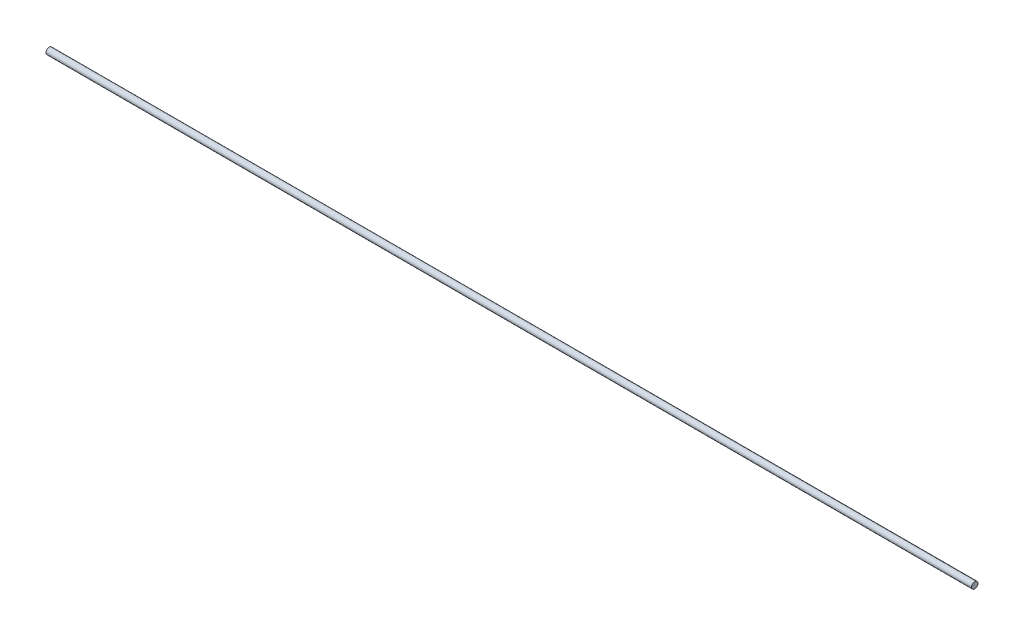
from build123d import *

# Parameters (mm, degrees)
SKETCH_1_W = 1440
SKETCH_1_H = 5


with BuildPart() as part:
    # 草图1 → 旋转1 (revolve)
    with BuildSketch(Plane.XY, mode=Mode.PRIVATE) as revolve_1_sk:
        with Locations((720, 47.5)):
            Rectangle(SKETCH_1_W, SKETCH_1_H)
    revolve(revolve_1_sk.sketch.rotate(Axis((0, 45, 0), (1, 0, 0)), 270), axis=Axis((0, 45, 0), (1, 0, 0)))


solid = part.part
